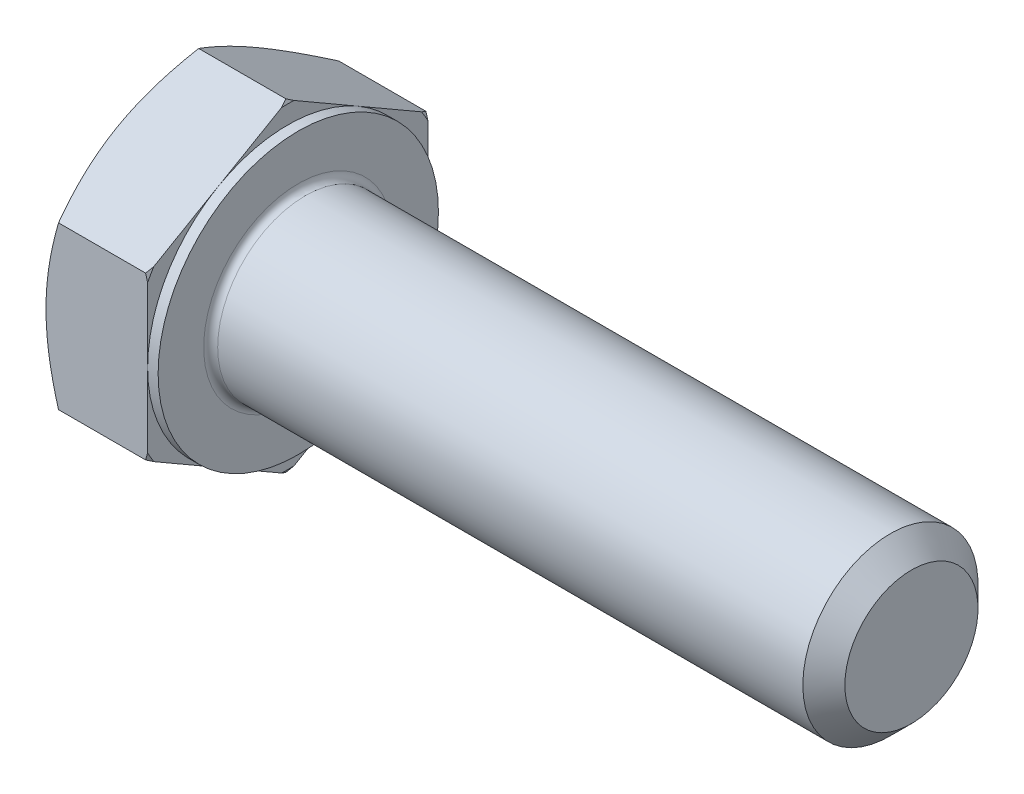
SolidWorks part; units mm, degrees
extrude "基体-拉伸" add sketch "草图1" along normal blind 6.4
sketch "草图1" plane through (0, 0, 0) normal (1, 0, 0) x (0, 0, -1)
  line L0 (8, 4.6188) -> (8, -4.6188)
  line L1 (-8, 4.6188) -> (-8, -4.6188)
  line L2 (8, -4.6188) -> (0, -9.2376)
  line L3 (0, -9.2376) -> (-8, -4.6188)
  line L4 (8, 4.6188) -> (0, 9.2376)
  line L5 (0, 9.2376) -> (-8, 4.6188)
revolve "切除-旋转1" cut sketch "草图3" angle 360 about L6
sketch "草图3" plane through (0, 0, 0) normal (0, 0, 1) x (1, 0, 0)
  line L0 (0, 8) -> (3.6013, 14.2376)
  line L1 (0, 9.2376) -> (0, 4.6188) construction
  line L2 (3.6013, 14.2376) -> (3.6013, 19.2376)
  line L3 (3.6013, 19.2376) -> (-10, 19.2376)
  line L4 (-10, 19.2376) -> (-10, 8)
  line L5 (-10, 8) -> (0, 8)
  line L6 (0, 0) -> (99.06, 0) construction
  line L7 (6.4, 9.2376) -> (0, 9.2376) construction
revolve "凸台-旋转1" add sketch "草图2" angle 360 about L7
sketch "草图2" plane through (0, 0, 0) normal (0, 0, 1) x (1, 0, 0)
  line L0 (0, 4.6188) -> (0, -4.6188) construction
  line L1 (0, 0) -> (41.4, 0)
  line L2 (0, 0) -> (0, 5)
  line L3 (0, 5) -> (41.4, 5)
  line L4 (41.4, 0) -> (41.4, 3.701)
  line L5 (6.4, 9.2376) -> (6.4, 4.6188) construction
  line L7 (0, 0) -> (96.52, 0) construction
  line L8 (41.4, -3.701) -> (90.335, -5) construction
  line L9 (0, -5) -> (90.335, -5) construction
  line L10 (7.9, 15.24) -> (7.9, -1.27) construction
  line L11 (6.4, 15.24) -> (6.4, -1.27) construction
  line L12 (6.4, 4.6188) -> (6.4, -4.6188) construction
  line L14 (41.4, 5) -> (41.4, 3.701)
  dimension "l" = 35
  dimension "m" = 10
  dimension "Minor_dia" = 7.402
  dimension "p" = 1.5
  dimension "h" = 35
cosmetic thread "螺旋线1" parameters "Thread_length"=33.5, "Thread_minor"=7.402
material "3.6级"
ref_plane "前视" through (0, 0, 0) normal (0, 0, 1) x (1, 0, 0)
ref_plane "上视" through (0, 0, 0) normal (0, 1, 0) x (1, 0, 0)
ref_plane "右视" through (0, 0, 0) normal (1, 0, 0) x (0, 0, -1)
sketch "草图5" plane through (0, 0, 0) normal (0, 0, 1) x (1, 0, 0)
  line L0 (6.4, 8) -> (2.7987, 14.2376)
  line L1 (6.4, 9.2376) -> (6.4, 4.6188) construction
  line L2 (2.7987, 14.2376) -> (2.7987, 19.2376)
  line L3 (2.7987, 19.2376) -> (12.7987, 19.2376)
  line L4 (12.7987, 19.2376) -> (12.7987, 8)
  line L5 (12.7987, 8) -> (6.4, 8)
  line L7 (6.4, 9.2376) -> (0.7145, 9.2376) construction
  line L8 (0, 0) -> (99.06, 0) construction
  line L9 (0, 0) -> (99.06, 0) construction
revolve "切除-旋转2" cut sketch "草图5" angle 360 about L8
sketch "草图4" plane through (0, 0, 0) normal (0, 0, 1) x (1, 0, 0)
  line L1 (6.4, 9.2376) -> (6.4, 4.6188) construction
  line L2 (6.4, 8) -> (5.8, 8)
  line L3 (6.4, 8) -> (6.4, 19.2376)
  line L4 (6.4, 19.2376) -> (5.8, 19.2376)
  line L5 (0, 0) -> (95.25, 0) construction
  line L6 (0, 0) -> (96.52, 0) construction
  line L7 (5.8, 8) -> (5.8, 19.2376)
  line L8 (5.6855, 9.2376) -> (0.7145, 9.2376) construction
revolve "切除-旋转3" cut sketch "草图4" angle 360 about L5
chamfer "倒角" distance 1.2 angle 45 1 edges at (41.4, 0, 5)
fillet "圆角" radius 0.4 1 edges at (6.4, 0, -5)
sketch "草图6" plane through (0, 0, 0) normal (0, 0, 1) x (1, 0, 0)
  line L0 (7.55, -3.701) -> (6.8, -5)
  line L1 (7.55, -3.701) -> (8.3, -5)
  line L2 (8.3, -5) -> (8.3, -6.25)
  line L3 (-3.175, 0) -> (5.1513, 0) construction
  line L5 (8.3, -6.25) -> (6.8, -6.25)
  line L6 (6.8, -6.25) -> (6.8, -5)
  arc A0 (6.8, -5) -> (6.4, -5.4) centre (6.8, -5.4) ccw construction
revolve "切除-旋转4" [suppressed] cut sketch "草图6" angle 360 about L3
pattern_linear "阵列(线性)1" [suppressed]
equation "\"D3@草图1\" = \"s@草图1\" / 2"
equation "\"D4@草图1\" = \"D3@草图1\""
equation "\"D5@草图1\" = \"D4@草图1\""
equation "\"D1@草图3\" = \"s@草图1\" / 2"
equation "\"D1@草图5\" = \"s@草图1\" / 2"
equation "\"Head_ch_ang@草图5\" = \"Head_ch_ang@草图3\""
equation "\"D1@草图4\" = \"s@草图1\""
equation "\"Diameter@草图6\" = \"m@草图2\""
equation "\"Overcut@草图6\" = \"m@草图2\" * 1.25"
equation "\"Minor_dia@草图2\" = \"m@草图2\"-\"p@草图2\" * 1.732"
equation "\"Thread_minor@螺旋线1\" = \"Minor_dia@草图2\""
equation "\"Thread_minor@草图6\" = \"Minor_dia@草图2\""
equation "\"D1@倒角\" = \"p@草图2\"*0.8"
equation "\"Thread_length@螺旋线1\" = \"l@草图2\" - \"p@草图2\""
equation "\"Num_threads@阵列(线性)1\" = \"l@草图2\" / \"p@草图2\""
